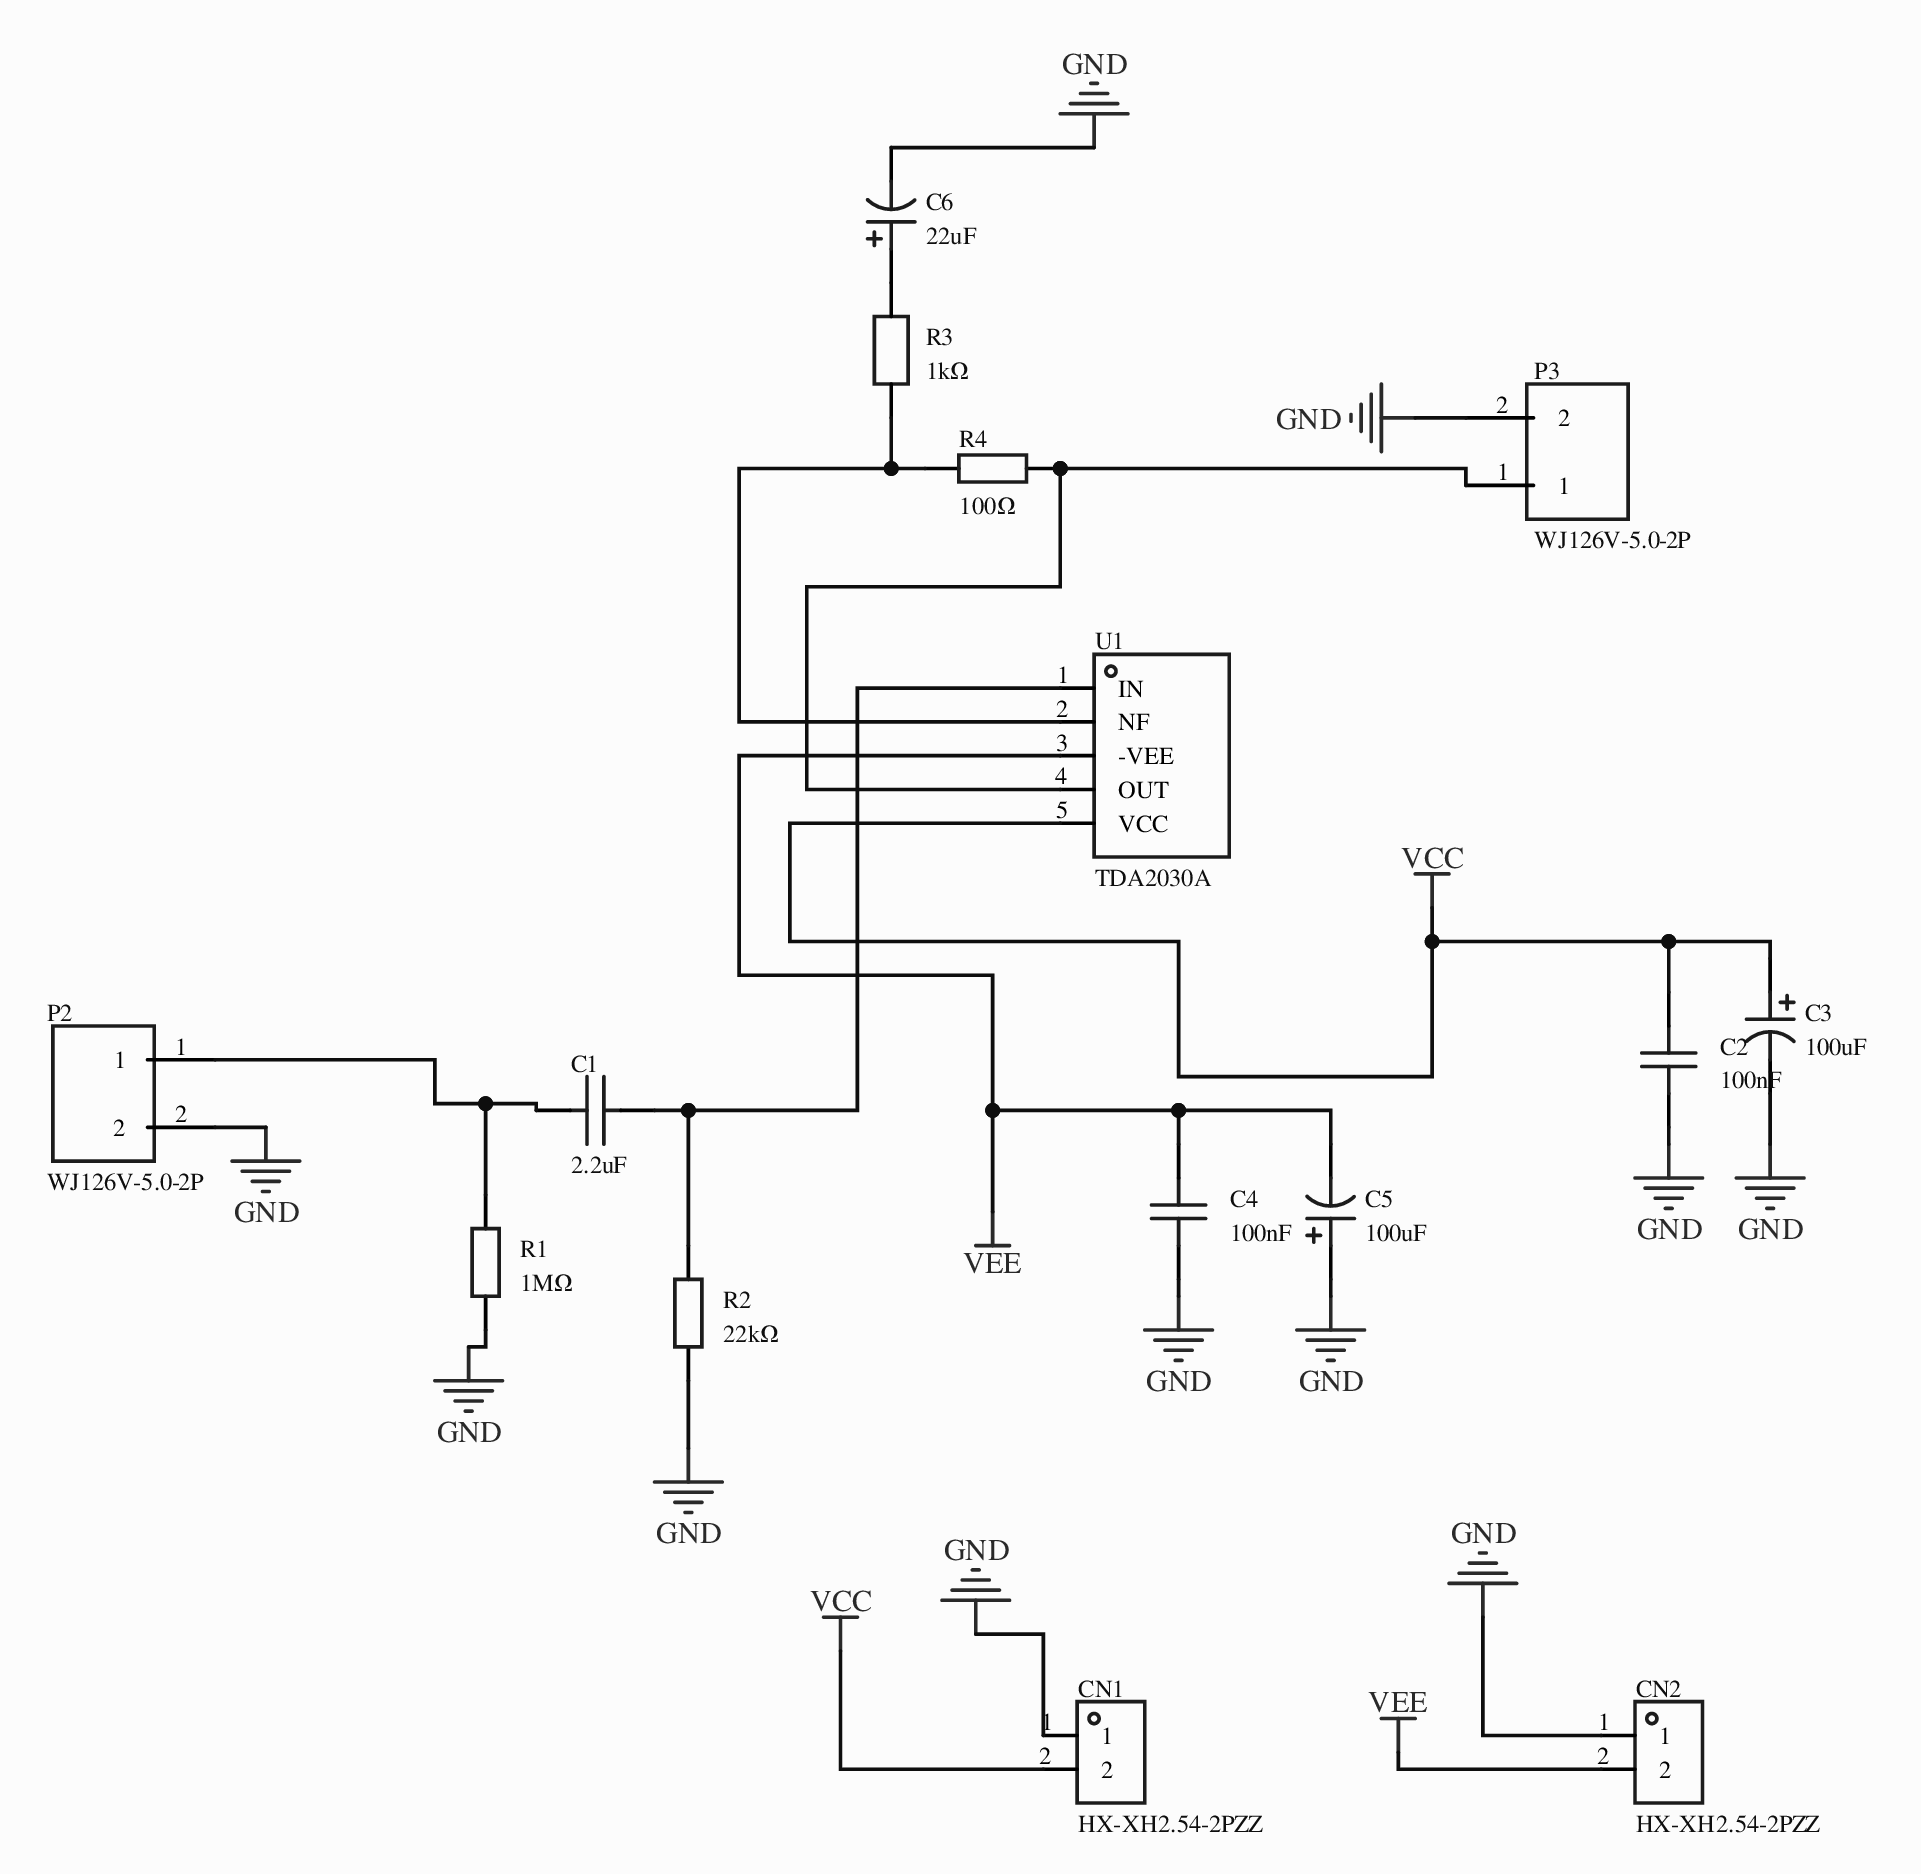
[diagram p0: MISC82886-3.schdoc]
# Altium project MISC82886.PrjPcb
1 sheet, 15 parts. Net scope: global (net labels, ports and power ports of the same name join across sheets).
Board file: MISC82886.pcbdoc

## Sheet MISC82886-3.schdoc
size 292 x 193 mm; Name: MISC82886

### Parts
C1  2.2uF  [C0402]
C2  100nF  [C0603]
C3  100uF  [CAP-TH_BD8.0-P3.50-D0.5-FD]
C4  100nF  [C0603]
C5  100uF  [CAP-TH_BD8.0-P3.50-D0.5-FD]
C6  22uF  [CAP-TH_BD10.0-P5.00-D0.6-FD]
CN1  HX-XH2.54-2PZZ  [CONN-TH_2P-P2.50_HX-2.54MM-2P-ZZ-MS]
CN2  HX-XH2.54-2PZZ  [CONN-TH_2P-P2.50_HX-2.54MM-2P-ZZ-MS]
P2  WJ126V-5.0-2P  [CONN-TH_WJ126V-5.0-2P]
P3  WJ126V-5.0-2P  [CONN-TH_WJ126V-5.0-2P]
R1  1MΩ  [R0603]
R2  22kΩ  [R0603]
R3  1kΩ  [R0603]
R4  100Ω  [R0805]
U1  TDA2030A  [TO-220B-5_L10.6-W8.7-P1.70-BL]

### Nets
GND: C2.1 C3.2 C4.1 C5.1 C6.2 CN1.1 CN2.1 P2.2 P3.2 R1.1 R2.1
VCC: C2.2 C3.1 CN1.2 U1.5(VCC)
VEE: C4.2 C5.2 CN2.2 U1.3(-VEE)
NetC1_1: C1.1 P2.1 R1.2
NetC1_2: C1.2 R2.2 U1.1(IN)
NetC6_1: C6.1 R3.2
NetP3_1: P3.1 R4.2 U1.4(OUT)
NetR3_1: R3.1 R4.1 U1.2(NF)

### Library data of the parts
C1 = CL05A225MQ5NSNC: Capacitance:2.2uF;Tolerance:±20%;Rated voltage:6.3V;Temperature coefficient:X5R;; Manufacturer: SAMSUNG(三星); AddInBom: yes; ModelId: 36a51122f27c49738f86b3bfa98863e00819f05c4eef4c71ace90d822a990e87; ModelName: C0402_L1.0-W0.5-H0.5; ModelTransform: 39.37,19.685,0,0,0,0,0,0,0; Tolerance: ±20%; Voltage Rating: 6.3V; Temperature Coefficient: X5R; Symbol: CL05A225MQ5NSNC; Device: CL05A225MQ5NSNC; LCSC Part Name: 2.2uF ±20% 6.3V; SupplierPart: C12530; ManufacturerPart: CL05A225MQ5NSNC; Supplier Footprint: 0402; JLCPCB Part Class: Basic Part; Datasheet: example.com/datasheet/CL05A225MQ5NSNC/13164.html; Supplier: LCSC; ConvertToPcb: yes; FootprintName: C0402; Value: 2.2uF
C2 C4 = CGA0603X7R104K500JT: Capacitance:100nF;Tolerance:±10%;Rated voltage:50V;Temperature coefficient:X7R;; Manufacturer: HRE(芯声); AddInBom: yes; ModelId: ac125912035d415993ca9572d50418b10819f05c4eef4c71ace90d822a990e87; ModelName: C0603_L1.6-W0.8-H0.8; ModelTransform: 62.992,31.496,0,0,0,0,0,0,0; Tolerance: ±10%; Voltage Rating: 50V; Temperature Coefficient: X7R; Symbol: CGA0603X7R104K500JT; Device: CGA0603X7R104K500JT; LCSC Part Name: 100nF ±10% 50V; SupplierPart: C6119867; ManufacturerPart: CGA0603X7R104K500JT; Supplier Footprint: 0603; JLCPCB Part Class: Extended Part; Datasheet: example.com/datasheet/CGA0603X7R104K500JT/7062573.html; Supplier: LCSC; ConvertToPcb: yes; FootprintName: C0603; Value: 100nF
C3 C5 = ERG50V100M8X12: Capacitance:100uF;Tolerance:±20%;Rated voltage:50V;Ripple current:680mA@100kHz;Equivalent series resistance(ESR):120mΩ@100kHz;; Manufacturer: JIERR(捷而瑞); AddInBom: yes; ModelId: 627d55c9ca1c4b51a61bba7c83a7ae6f0819f05c4eef4c71ace90d822a990e87; ModelTransform: 314.96,315.3537,0,90,0,0,0,0,-196.85; Tolerance: ±20%; Voltage Rating: 50V; Pin Spacing: 3.5mm; Lifetime: 2000hrs@105℃; Symbol: ERG50V100M8X12; Device: ERG50V100M8X12; LCSC Part Name: 100uF ±20% 50V; SupplierPart: C47344183; ManufacturerPart: ERG50V100M8X12; Supplier Footprint: 插件,D8xL12mm; JLCPCB Part Class: Extended Part; Datasheet: example.com/datasheet/ERG50V100M8X12/49556624.html; Supplier: LCSC; ConvertToPcb: yes; FootprintName: CAP-TH_BD8.0-P3.50-D0.5-FD; ModelName: CAP-TH_BD8.0-P3.50-D0.5-FD; Value: 100uF; Ripple Current: 680mA@100kHz; Equivalent Series Resistance(ESR): 120mΩ@100kHz; Diameter: 8mm; Height - Seated (Max): 12mm; Operating Temperature: -40℃~+105℃
C6 = ERG400V22M10X17: Capacitance:22uF;Tolerance:±20%;Rated voltage:400V;Ripple current:145mA@100kHz;Equivalent series resistance(ESR):7.8Ω@100kHz;; Manufacturer: JIERR(捷而瑞); AddInBom: yes; ModelId: e69a8877034041adb17289105fbfdf3e0819f05c4eef4c71ace90d822a990e87; ModelTransform: 394.094,393.211,0,0,0,0,-0.005,0,-137.795; Tolerance: ±20%; Voltage Rating: 400V; Pin Spacing: 5mm; Lifetime: 3000hrs@105℃; Symbol: ERG400V22M10X17; Device: ERG400V22M10X17; LCSC Part Name: 22uF ±20% 400V; SupplierPart: C51904441; ManufacturerPart: ERG400V22M10X17; Supplier Footprint: 插件,D10xL17mm; JLCPCB Part Class: Extended Part; Datasheet: example.com/datasheet/ERG400V22M10X17/54596810.html; Supplier: LCSC; ConvertToPcb: yes; FootprintName: CAP-TH_BD10.0-P5.00-D0.6-FD; ModelName: CAP-TH_BD10.0-P5.00-D0.6-FD; Value: 22uF; Ripple Current: 145mA@100kHz; Equivalent Series Resistance(ESR): 7.8Ω@100kHz; Diameter: 10mm; Height - Seated (Max): 17mm; Operating Temperature: -25℃~+105℃
CN1 CN2 = HX-XH2.54-2PZZ: Pin structure:1x2P;Pitch:2.54mm;Mounting:through-hole;Reference series:XH;Total pins:2P;Rows:1;Pins per row:2;Row spacing:-;Rated current:3A;Contact material:brass;Contact plating:tin;Working temperature:-25℃~+85℃;; Manufacturer: hanxia(韩下); AddInBom: yes; ModelId: 1cafe43f43c04794b29c478db770ea2f0819f05c4eef4c71ace90d822a990e87; ModelTransform: 295.275,228.7397,0,0,0,0,0,-19.685,-137.795; Pins Structure: 1x2P; Pitch: 2.54mm; Reference Series: XH; Number of PINs Per Row: 2; Current Rating: 3A; Voltage Rating: 250V; Plastic Material: PA66; Flame Retardant Rating: UL94V-0; Symbol: HX-XH2.54-2PZZ; Device: HX-XH2.54-2PZZ; LCSC Part Name: 1x2P 间距:2.5mm 直插 系列:XH; SupplierPart: C42391660; ManufacturerPart: HX-XH2.54-2PZZ; Supplier Footprint: 插件,P=2.5mm; JLCPCB Part Class: Extended Part; Datasheet: example.com/datasheet/HX-XH2.54-2PZZ/44326932.html; Supplier: LCSC; ConvertToPcb: yes; FootprintName: CONN-TH_2P-P2.50_HX-2.54MM-2P-ZZ-MS; ModelName: CONN-TH_2P-P2.50_HX-2.54MM-2P-ZZ-MS; Mounting Type: through-hole; Number of Pins: 2P; Number of Rows: 1; Row Spacing: -; Contact Material: Brass; Contact Plating: tin; Operating Temperature: -25℃~+85℃; Color: white
P2 P3 = WJ126V-5.0-2P: Structure:1x2P;Pitch:5mm;Colour:green;Mounting:through-hole;Rows:1;Pins per row:2;Rated current:18A;Rated voltage:250V;Wire gauge - AWG:14~26;Wire gauge - sq mm:2.5;Working temperature:-40℃~+105℃;; Manufacturer: KANGNEX(康奈克斯电气); AddInBom: yes; ModelId: 7b5c7c9de40d47b68e660a99957f0f3e0819f05c4eef4c71ace90d822a990e87; ModelName: CONN-TH_DB5.00-LI-2P-126; ModelTransform: 410.149,307.086,0,90,0,0,3.937,9.842,-137.795; Number of Positions or Pins: 1x2P; Pitch: 5mm; Number of PINs Per Row: 2; Current Rating: 18A; Voltage Rating (Max): 250V; Wire Gauge - AWG: 14~26; Wire Gauge - mm2: 2.5; Symbol: WJ126V-5.0-2P; Device: WJ126V-5.0-2P; LCSC Part Name: 5mm 1x2P 排数:1 每排P数:2 直插; SupplierPart: C8404; ManufacturerPart: WJ126V-5.0-2P; Supplier Footprint: 插件,P=5mm; JLCPCB Part Class: Extended Part; Datasheet: example.com/datasheet/WJ126V-5.0-2P/8898.html; Supplier: LCSC; ConvertToPcb: yes; FootprintName: CONN-TH_WJ126V-5.0-2P; Color: green; Mounting Type: through-hole; Number of Pins: 2P; Number of Rows: 1; Operating Temperature: -40℃~+105℃
R1 = 0603WAF1004T5E: Resistor type:thick film;Resistance:1MΩ;Tolerance:±1%;Power:100mW;Max working voltage:75V;Temperature coefficient:±100ppm/℃;; Manufacturer: UNI-ROYAL(厚声); AddInBom: yes; ModelId: fc143cca1e79419f9cd78b61e9279f080819f05c4eef4c71ace90d822a990e87; ModelTransform: 31.8897,63.7794,0,90,0,0,0,0,0; Tolerance: ±1%; Power(Watts): 100mW; Overload Voltage (Max): 75V; Symbol: 0603WAF1004T5E; Device: 0603WAF1004T5E; LCSC Part Name: 1MΩ ±1% 100mW 厚膜电阻; SupplierPart: C22935; ManufacturerPart: 0603WAF1004T5E; Supplier Footprint: 0603; JLCPCB Part Class: Basic Part; Datasheet: example.com/upload/public/pdf/source/20200306/C422600_1E6D84923E4A46A82E41ADD87F860B5C.pdf; Supplier: LCSC; ConvertToPcb: yes; FootprintName: R0603; ModelName: R0603; Type: thick film; Value: 1MΩ; Temperature Coefficient: ±100ppm/℃; Operating Temperature Range: -55℃~+155℃
R2 = 0603WAF2202T5E: Resistor type:thick film;Resistance:22kΩ;Tolerance:±1%;Power:100mW;Working voltage:75V;Temperature coefficient:±100ppm/℃;; Manufacturer: UNI-ROYAL(厚声); AddInBom: yes; ModelId: fc143cca1e79419f9cd78b61e9279f080819f05c4eef4c71ace90d822a990e87; ModelTransform: 31.8897,63.7794,0,90,0,0,0,0,0; Tolerance: ±1%; Power(Watts): 100mW; Voltage-Supply(Max): 75V; Symbol: 0603WAF2202T5E; Device: 0603WAF2202T5E; LCSC Part Name: 22kΩ ±1% 100mW 厚膜电阻; SupplierPart: C31850; ManufacturerPart: 0603WAF2202T5E; Supplier Footprint: 0603; JLCPCB Part Class: Basic Part; Datasheet: example.com/datasheet/0603WAF2202T5E/32812.html; Supplier: LCSC; ConvertToPcb: yes; FootprintName: R0603; ModelName: R0603; Type: thick film; Value: 22kΩ; Temperature Coefficient: ±100ppm/℃; Operating Temperature: -55℃~+155℃
R3 = FRC0603F1001TS: Resistor type:thick film;Resistance:1kΩ;Tolerance:±1%;Power:100mW;Working voltage:75V;Temperature coefficient:±100ppm/℃;; Manufacturer: FOJAN(富捷); AddInBom: yes; ModelId: fc143cca1e79419f9cd78b61e9279f080819f05c4eef4c71ace90d822a990e87; ModelTransform: 31.8897,63.7794,0,90,0,0,0,0,0; Tolerance: ±1%; Power(Watts): 100mW; Voltage-Supply(Max): 75V; Symbol: FRC0603F1001TS; Device: FRC0603F1001TS; LCSC Part Name: 1kΩ ±1% 100mW 厚膜电阻; SupplierPart: C2907002; ManufacturerPart: FRC0603F1001TS; Supplier Footprint: 0603; JLCPCB Part Class: Extended Part; Supplier: LCSC; ConvertToPcb: yes; FootprintName: R0603; ModelName: R0603; Type: thick film; Value: 1kΩ; Temperature Coefficient: ±100ppm/℃; Operating Temperature: -55℃~+155℃
R4 = 0805W8F1000T5E: Resistor type:thick film;Resistance:100Ω;Tolerance:±1%;Power:125mW;Max working voltage:150V;Temperature coefficient:±100ppm/℃;; Manufacturer: UNI-ROYAL(厚声); AddInBom: yes; ModelId: 37a81e68749a4138bd2dfa6897b24b850819f05c4eef4c71ace90d822a990e87; ModelName: R0805_L2.0-W1.3-H0.6; ModelTransform: 78.74,51.181,0,0,0,0,0,-0.0005,0; Tolerance: ±1%; Power(Watts): 125mW; Overload Voltage (Max): 150V; Symbol: 0805W8F1000T5E; Device: 0805W8F1000T5E; LCSC Part Name: 100Ω ±1% 125mW 厚膜电阻; SupplierPart: C17408; ManufacturerPart: 0805W8F1000T5E; Supplier Footprint: 0805; JLCPCB Part Class: Basic Part; Datasheet: example.com/upload/public/pdf/source/20200306/C422600_1E6D84923E4A46A82E41ADD87F860B5C.pdf; Supplier: LCSC; ConvertToPcb: yes; FootprintName: R0805; Type: thick film; Value: 100Ω; Temperature Coefficient: ±100ppm/℃; Operating Temperature Range: -55℃~+155℃
U1 = TDA2030A: Amplifier type:-;Speaker channels:mono;Output power:18W;Quiescent current(Iq):40mA;; Manufacturer: minos(迈诺斯); AddInBom: yes; ModelId: df4891f36111459a820b14d5b303e2980819f05c4eef4c71ace90d822a990e87; ModelTransform: 399.999,330.74737,0,0,0,0,0,80.787,-196.85; Speaker Channels: mono; Output Power: 18W; Total Harmonic Distortion + Noise (THD+N): 0.2%; Quiescent Current: 40mA; Power Supply Rejection Ratio (PSRR): 50dB; Voltage - Supply: 6V~18V; Symbol: TDA2030A; Device: TDA2030A; LCSC Part Name: 18W 音频功率放大电路; SupplierPart: C5121614; ManufacturerPart: TDA2030A; Supplier Footprint: TO-220B-5; JLCPCB Part Class: Extended Part; Datasheet: example.com/datasheet/TDA2030A/5709493.html; Supplier: LCSC; ConvertToPcb: yes; FootprintName: TO-220B-5_L10.6-W8.7-P1.70-BL; ModelName: TO-220B-5_L10.6-W8.7-P1.70-BL; Class: -; Signal-to-Noise Ratio: -; Efficiency: -; Number of Inputs: -; Features: -; Operating Temperature: -20℃~+75℃